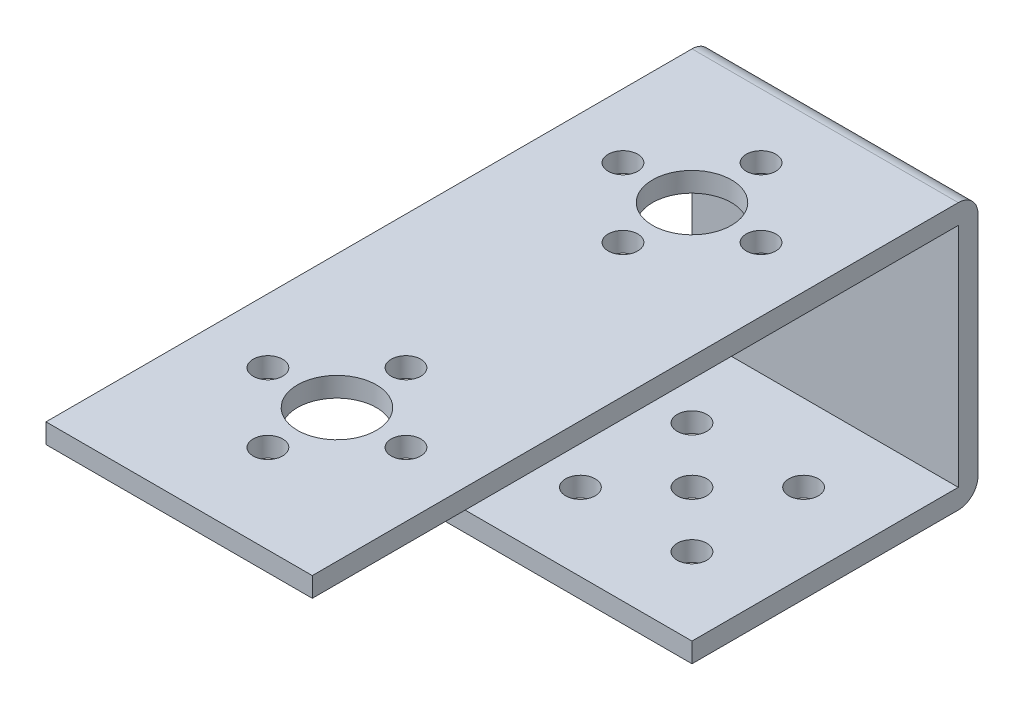
from build123d import *

# Parameters (mm, degrees)
SKETCH1_W           = 27
SKETCH1_H           = 27
BOSS_EXTRUDE1_DEPTH = 29
SKETCH2_W           = 27
SKETCH2_H           = 23
CUT_EXTRUDE1_DEPTH  = 27
CUT_EXTRUDE2_REACH  = 43.86
SKETCH4_R           = 4
SKETCH4_R_2         = 1.5
CUT_EXTRUDE3_REACH  = 43.86
SKETCH5_R           = 1.5
FILLET1_R           = 2
SKETCH6_W           = 27
SKETCH6_H           = 2
BOSS_EXTRUDE2_DEPTH = 38.5
SKETCH7_R           = 4
SKETCH7_R_2         = 1.5
CUT_EXTRUDE4_DEPTH  = 2


with BuildPart() as part:
    # Sketch1 → Boss-Extrude1 (new body)
    with BuildSketch(Plane.XY):
        Rectangle(SKETCH1_W, SKETCH1_H)
    extrude(amount=BOSS_EXTRUDE1_DEPTH)

    # Sketch2 → Cut-Extrude1 (cut)
    with BuildSketch(Plane(origin=(13.5, 0, 0), x_dir=(0, 0, -1), z_dir=(1, 0, 0))):
        with Locations((-15.5, 0)):
            Rectangle(SKETCH2_W, SKETCH2_H)
    extrude(amount=-CUT_EXTRUDE1_DEPTH, mode=Mode.SUBTRACT)

    # Sketch4 → Cut-Extrude2 (cut, up to next)
    with BuildSketch(Plane(origin=(0, 13.5, 0), x_dir=(1, 0, 0), z_dir=(0, 1, 0)), mode=Mode.PRIVATE) as cut_extrude2_sk1:
        with Locations(Location((0, -15.5, 0), (0, 0, 270))):
            Circle(SKETCH4_R)
    cut_extrude2_tool1 = extrude(cut_extrude2_sk1.sketch, amount=-CUT_EXTRUDE2_REACH, mode=Mode.PRIVATE) & part.part
    # Sketch4 → Cut-Extrude2 (cut, up to next)
    with BuildSketch(Plane(origin=(0, 13.5, 0), x_dir=(1, 0, 0), z_dir=(0, 1, 0)), mode=Mode.PRIVATE) as cut_extrude2_sk2:
        with Locations(Location((0, -8.5, 0), (0, 0, 270))):
            Circle(SKETCH4_R_2)
    cut_extrude2_tool2 = extrude(cut_extrude2_sk2.sketch, amount=-CUT_EXTRUDE2_REACH, mode=Mode.PRIVATE) & part.part
    # Sketch4 → Cut-Extrude2 (cut, up to next)
    with BuildSketch(Plane(origin=(0, 13.5, 0), x_dir=(1, 0, 0), z_dir=(0, 1, 0)), mode=Mode.PRIVATE) as cut_extrude2_sk3:
        with Locations(Location((7, -15.5, 0), (0, 0, 270))):
            Circle(SKETCH4_R_2)
    cut_extrude2_tool3 = extrude(cut_extrude2_sk3.sketch, amount=-CUT_EXTRUDE2_REACH, mode=Mode.PRIVATE) & part.part
    # Sketch4 → Cut-Extrude2 (cut, up to next)
    with BuildSketch(Plane(origin=(0, 13.5, 0), x_dir=(1, 0, 0), z_dir=(0, 1, 0)), mode=Mode.PRIVATE) as cut_extrude2_sk4:
        with Locations(Location((0, -22.5, 0), (0, 0, 270))):
            Circle(SKETCH4_R_2)
    cut_extrude2_tool4 = extrude(cut_extrude2_sk4.sketch, amount=-CUT_EXTRUDE2_REACH, mode=Mode.PRIVATE) & part.part
    # Sketch4 → Cut-Extrude2 (cut, up to next)
    with BuildSketch(Plane(origin=(0, 13.5, 0), x_dir=(1, 0, 0), z_dir=(0, 1, 0)), mode=Mode.PRIVATE) as cut_extrude2_sk5:
        with Locations(Location((-7, -15.5, 0), (0, 0, 270))):
            Circle(SKETCH4_R_2)
    cut_extrude2_tool5 = extrude(cut_extrude2_sk5.sketch, amount=-CUT_EXTRUDE2_REACH, mode=Mode.PRIVATE) & part.part
    add(cut_extrude2_tool1.solids().sort_by_distance((0, 13.5, 15.5))[0], mode=Mode.SUBTRACT)
    add(cut_extrude2_tool2.solids().sort_by_distance((0, 13.5, 8.5))[0], mode=Mode.SUBTRACT)
    add(cut_extrude2_tool3.solids().sort_by_distance((7, 13.5, 15.5))[0], mode=Mode.SUBTRACT)
    add(cut_extrude2_tool4.solids().sort_by_distance((0, 13.5, 22.5))[0], mode=Mode.SUBTRACT)
    add(cut_extrude2_tool5.solids().sort_by_distance((-7, 13.5, 15.5))[0], mode=Mode.SUBTRACT)

    # Sketch5 → Cut-Extrude3 (cut, up to next)
    with BuildSketch(Plane.XZ.offset(13.5), mode=Mode.PRIVATE) as cut_extrude3_sk1:
        with Locations(Location((0, 15.5, 0), (0, 0, 270))):
            Circle(SKETCH5_R)
    cut_extrude3_tool1 = extrude(cut_extrude3_sk1.sketch, amount=-CUT_EXTRUDE3_REACH, mode=Mode.PRIVATE) & part.part
    # Sketch5 → Cut-Extrude3 (cut, up to next)
    with BuildSketch(Plane.XZ.offset(13.5), mode=Mode.PRIVATE) as cut_extrude3_sk2:
        with Locations(Location((-5.656854249, 21.156854249, 0), (0, 0, 270))):
            Circle(SKETCH5_R)
    cut_extrude3_tool2 = extrude(cut_extrude3_sk2.sketch, amount=-CUT_EXTRUDE3_REACH, mode=Mode.PRIVATE) & part.part
    # Sketch5 → Cut-Extrude3 (cut, up to next)
    with BuildSketch(Plane.XZ.offset(13.5), mode=Mode.PRIVATE) as cut_extrude3_sk3:
        with Locations(Location((5.656854249, 21.156854249, 0), (0, 0, 270))):
            Circle(SKETCH5_R)
    cut_extrude3_tool3 = extrude(cut_extrude3_sk3.sketch, amount=-CUT_EXTRUDE3_REACH, mode=Mode.PRIVATE) & part.part
    # Sketch5 → Cut-Extrude3 (cut, up to next)
    with BuildSketch(Plane.XZ.offset(13.5), mode=Mode.PRIVATE) as cut_extrude3_sk4:
        with Locations(Location((5.656854249, 9.843145751, 0), (0, 0, 270))):
            Circle(SKETCH5_R)
    cut_extrude3_tool4 = extrude(cut_extrude3_sk4.sketch, amount=-CUT_EXTRUDE3_REACH, mode=Mode.PRIVATE) & part.part
    # Sketch5 → Cut-Extrude3 (cut, up to next)
    with BuildSketch(Plane.XZ.offset(13.5), mode=Mode.PRIVATE) as cut_extrude3_sk5:
        with Locations(Location((-5.656854249, 9.843145751, 0), (0, 0, 270))):
            Circle(SKETCH5_R)
    cut_extrude3_tool5 = extrude(cut_extrude3_sk5.sketch, amount=-CUT_EXTRUDE3_REACH, mode=Mode.PRIVATE) & part.part
    add(cut_extrude3_tool1.solids().sort_by_distance((0, -13.5, 15.5))[0], mode=Mode.SUBTRACT)
    add(cut_extrude3_tool2.solids().sort_by_distance((-5.656854, -13.5, 21.156854))[0], mode=Mode.SUBTRACT)
    add(cut_extrude3_tool3.solids().sort_by_distance((5.656854, -13.5, 21.156854))[0], mode=Mode.SUBTRACT)
    add(cut_extrude3_tool4.solids().sort_by_distance((5.656854, -13.5, 9.843146))[0], mode=Mode.SUBTRACT)
    add(cut_extrude3_tool5.solids().sort_by_distance((-5.656854, -13.5, 9.843146))[0], mode=Mode.SUBTRACT)

    # Fillet1
    fillet1_edges = [part.edges().sort_by_distance(p)[0] for p in [
        (0, -13.5, 0),
        (0, 13.5, 0),
    ]]
    fillet(fillet1_edges, radius=FILLET1_R)

    # Sketch6 → Boss-Extrude2 (add)
    with BuildSketch(Plane.XY.offset(29)):
        with Locations((0, 12.5)):
            Rectangle(SKETCH6_W, SKETCH6_H)
    extrude(amount=BOSS_EXTRUDE2_DEPTH)

    # Sketch7 → Cut-Extrude4 (cut)
    with BuildSketch(Plane(origin=(0, 13.5, 0), x_dir=(1, 0, 0), z_dir=(0, 1, 0))):
        with Locations(Location((0, -51.5, 0), (0, 0, 270))):
            Circle(SKETCH7_R)
        with Locations(Location((0, -44.5, 0), (0, 0, 270))):
            Circle(SKETCH7_R_2)
        with Locations(Location((7, -51.5, 0), (0, 0, 270))):
            Circle(SKETCH7_R_2)
        with Locations(Location((0, -58.5, 0), (0, 0, 270))):
            Circle(SKETCH7_R_2)
        with Locations(Location((-7, -51.5, 0), (0, 0, 270))):
            Circle(SKETCH7_R_2)
    extrude(amount=-CUT_EXTRUDE4_DEPTH, mode=Mode.SUBTRACT)


solid = part.part
